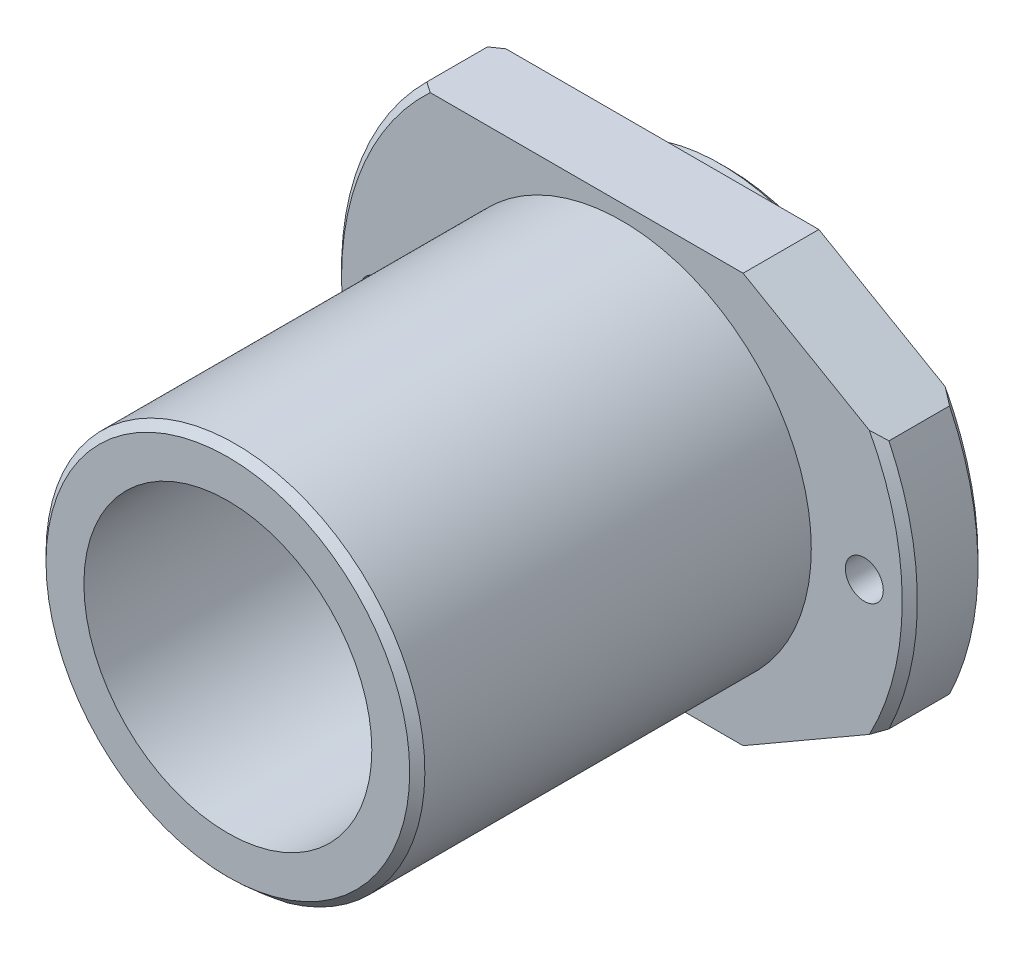
from build123d import *

# Parameters (mm, degrees)
SKETCH1_R             = 12.5
BOSS_EXTRUDE1_DEPTH   = 26
SKETCH2_R             = 19
BOSS_EXTRUDE2_DEPTH   = 5
BOSS_EXTRUDE3_START   = 2
SKETCH3_R             = 12.5
BOSS_EXTRUDE3_DEPTH   = 2
CHAMFER1_SIZE         = 0.5
SKETCH4_W             = 56.768050843
SKETCH4_H             = 11.338169824
SKETCH4_W_2           = 56.148312297
SKETCH4_H_2           = 14.587502032
CUT_EXTRUDE1_DEPTH    = 38.389838192
SKETCH5_R             = 9.5
CUT_EXTRUDE2_DEPTH    = 41.401113846
M3_TAPPED_HOLE1_D     = 2.5
M3_TAPPED_HOLE1_DEPTH = 7.5
M3_TAPPED_HOLE1_TIP   = 0.751075774
CUT_EXTRUDE3_DEPTH    = 10
SKETCH11_W            = 60.135329508
SKETCH11_H            = 29.448988524
CUT_EXTRUDE4_DEPTH    = 25


with BuildPart() as part:
    # Sketch1 → Boss-Extrude1 (new body)
    with BuildSketch(Plane.XY):
        with Locations(Location((0, 0, 0), (0, 0, 180))):
            Circle(SKETCH1_R)
    extrude(amount=BOSS_EXTRUDE1_DEPTH)

    # Sketch2 → Boss-Extrude2 (add)
    with BuildSketch(Plane(origin=(0, 0, 0), x_dir=(-1, 0, 0), z_dir=(0, 0, -1))):
        Circle(SKETCH2_R)
    extrude(amount=BOSS_EXTRUDE2_DEPTH)

    # Sketch3 → Boss-Extrude3 (add)
    with BuildSketch(Plane(origin=(0, 0, -5), x_dir=(-1, 0, 0), z_dir=(0, 0, -1)).offset(BOSS_EXTRUDE3_START)):
        Circle(SKETCH3_R)
    extrude(amount=-BOSS_EXTRUDE3_DEPTH)

    # Chamfer1
    chamfer1_edges = [part.edges().sort_by_distance(p)[0] for p in [
        (12.5, 0, -7),
        (12.5, 0, 26),
        (19, 0, 0),
        (19, 0, -5),
    ]]
    chamfer(chamfer1_edges, length=CHAMFER1_SIZE)

    # Sketch4 → Cut-Extrude1 (cut, through all)
    with BuildSketch(Plane.XY):
        with Locations((-0.433816982, -19.169084912)):
            Rectangle(SKETCH4_W, SKETCH4_H)
        with Locations((-0.743686256, 20.793751016)):
            Rectangle(SKETCH4_W_2, SKETCH4_H_2)
    extrude(amount=-CUT_EXTRUDE1_DEPTH, mode=Mode.SUBTRACT)

    # Sketch5 → Cut-Extrude2 (cut, through all)
    with BuildSketch(Plane.XY.offset(26)):
        Circle(SKETCH5_R)
    extrude(amount=-CUT_EXTRUDE2_DEPTH, mode=Mode.SUBTRACT)

    # M3 Tapped Hole1
    with Locations(Plane.XY):
        with Locations((16, 0), (-16, 0)):
            Hole(M3_TAPPED_HOLE1_D / 2, depth=M3_TAPPED_HOLE1_DEPTH)
            with Locations((0, 0, -(M3_TAPPED_HOLE1_DEPTH + M3_TAPPED_HOLE1_TIP / 2))):  # 118° drill point
                Cone(0, M3_TAPPED_HOLE1_D / 2, M3_TAPPED_HOLE1_TIP, mode=Mode.SUBTRACT)

    # Sketch10 → Cut-Extrude3 (cut)
    with BuildSketch(Plane.XY):
        Polygon((20.899032633, 6.052740037), (8, 13.5), (20.899032633, 13.5), align=None)
    cut_extrude3 = extrude(amount=-CUT_EXTRUDE3_DEPTH, mode=Mode.SUBTRACT)

    # Mirror1: Cut-Extrude3 across plane
    add(cut_extrude3.mirror(Plane.ZX), mode=Mode.SUBTRACT)

    # Sketch11 → Cut-Extrude4 (cut)
    with BuildSketch(Plane.XY.offset(26)):
        with Locations((5.227667093, -26.724494262)):
            Rectangle(SKETCH11_W, SKETCH11_H)
    extrude(amount=-CUT_EXTRUDE4_DEPTH, mode=Mode.SUBTRACT)


solid = part.part
